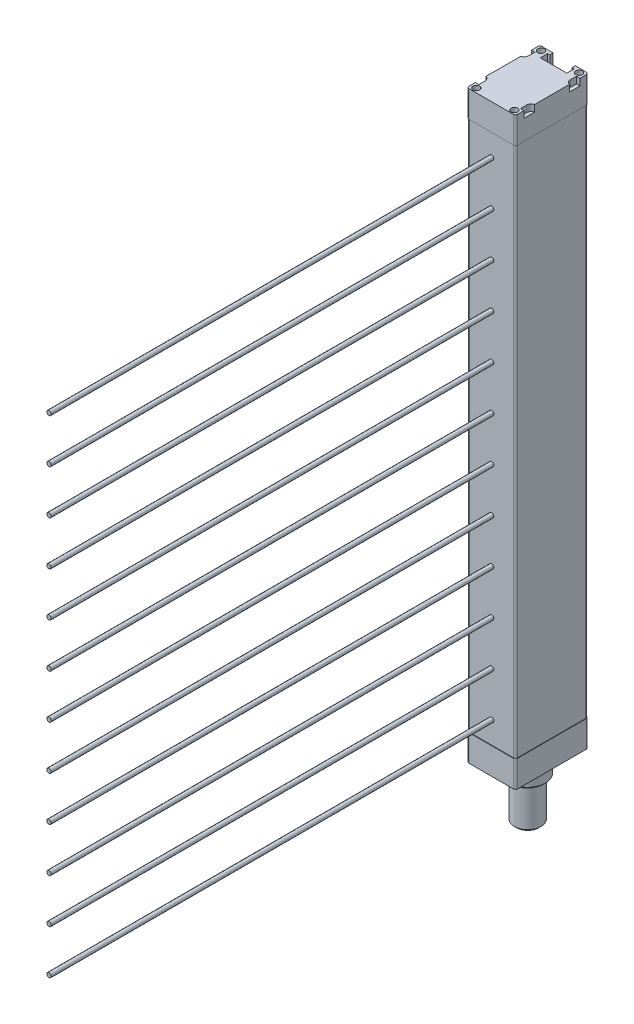
from build123d import *

# Parameters (mm, degrees)
SKETCH_1_R             = 1.5
EXTRUDE_1_DEPTH        = 12
CUT_EXTRUDE_2_DEPTH    = 3
EXTRUDE_3_DEPTH        = 240
SKETCH_5_R             = 1
EXTRUDE_4_DEPTH        = 200
PATTERN_LINEAR_1_COUNT = 12
PATTERN_LINEAR_1_PITCH = 20


with BuildPart() as part:
    # 草圖1 → 伸長1 (new body)
    with BuildSketch(Plane(origin=(0, 0, 0), x_dir=(1, 0, 0), z_dir=(0, 1, 0))):
        with BuildLine():
            Line((-10, 16.5), (-5, 16.5))
            Line((-5, 16.5), (-5, 15))
            Line((-5, 15), (-6, 15))
            Line((-6, 15), (-6, 11.7))
            Line((-6, 11.7), (6, 11.7))
            Line((6, 11.7), (6, 15))
            Line((6, 15), (5, 15))
            Line((5, 15), (5, 16.5))
            Line((5, 16.5), (10, 16.5))
            ThreePointArc((10, 16.5), (10.707106781, 16.207106781), (11, 15.5))
            Line((11, 15.5), (11, -15.5))
            ThreePointArc((11, -15.5), (10.707106781, -16.207106781), (10, -16.5))
            Line((10, -16.5), (-10, -16.5))
            ThreePointArc((-10, -16.5), (-10.707106781, -16.207106781), (-11, -15.5))
            Line((-11, -15.5), (-11, 15.5))
            ThreePointArc((-11, 15.5), (-10.707106781, 16.207106781), (-10, 16.5))
        make_face()
        with Locations(Location((-8.6, 14.6, 0), (0, 0, 270))):
            Circle(SKETCH_1_R, mode=Mode.SUBTRACT)
        with Locations(Location((8.6, 14.6, 0), (0, 0, 90))):
            Circle(SKETCH_1_R, mode=Mode.SUBTRACT)
        with Locations(Location((8.6, -14.6, 0), (0, 0, 270))):
            Circle(SKETCH_1_R, mode=Mode.SUBTRACT)
        with Locations(Location((-8.6, -14.6, 0), (0, 0, 90))):
            Circle(SKETCH_1_R, mode=Mode.SUBTRACT)
    extrude_1 = extrude(amount=EXTRUDE_1_DEPTH)

    # 草圖2 → 伸長2 (cut)
    with BuildSketch(Plane(origin=(0, 12, 0), x_dir=(1, 0, 0), z_dir=(0, 1, 0))):
        with BuildLine():
            Line((-14.2, 12.65), (-9.4, 12.65))
            Line((-9.4, 12.65), (-9.4, 9.85))
            ThreePointArc((-9.4, 9.85), (-9.985786438, 8.435786438), (-11.4, 7.85))
            Line((-11.4, 7.85), (-14.2, 7.85))
            Line((-14.2, 7.85), (-14.2, 12.65))
        make_face()
        with BuildLine():
            Line((9.4, 12.65), (9.4, 9.85))
            ThreePointArc((9.4, 9.85), (9.985786438, 8.435786438), (11.4, 7.85))
            Line((11.4, 7.85), (14.2, 7.85))
            Line((14.2, 7.85), (14.2, 12.65))
            Line((14.2, 12.65), (9.4, 12.65))
        make_face()
        with BuildLine():
            Line((14.2, -12.65), (9.4, -12.65))
            Line((9.4, -12.65), (9.4, -9.85))
            ThreePointArc((9.4, -9.85), (9.985786438, -8.435786438), (11.4, -7.85))
            Line((11.4, -7.85), (14.2, -7.85))
            Line((14.2, -7.85), (14.2, -12.65))
        make_face()
        with BuildLine():
            Line((-9.4, -12.65), (-9.4, -9.85))
            ThreePointArc((-9.4, -9.85), (-9.985786438, -8.435786438), (-11.4, -7.85))
            Line((-11.4, -7.85), (-14.2, -7.85))
            Line((-14.2, -7.85), (-14.2, -12.65))
            Line((-14.2, -12.65), (-9.4, -12.65))
        make_face()
    extrude(amount=-CUT_EXTRUDE_2_DEPTH, mode=Mode.SUBTRACT)

    # 草圖3 → 伸長3 (add)
    with BuildSketch(Plane.XZ):
        with BuildLine():
            Line((-5.2, -16.3), (-5.2, -15.2))
            Line((-5.2, -15.2), (-6.2, -15.2))
            Line((-6.2, -15.2), (-6.2, -11.5))
            Line((-6.2, -11.5), (6.2, -11.5))
            Line((6.2, -11.5), (6.2, -15.2))
            Line((6.2, -15.2), (5.2, -15.2))
            Line((5.2, -15.2), (5.2, -16.3))
            Line((5.2, -16.3), (10, -16.3))
            ThreePointArc((10, -16.3), (10.565685425, -16.065685425), (10.8, -15.5))
            Line((10.8, -15.5), (10.8, 15.5))
            ThreePointArc((10.8, 15.5), (10.565685425, 16.065685425), (10, 16.3))
            Line((10, 16.3), (-10, 16.3))
            ThreePointArc((-10, 16.3), (-10.565685425, 16.065685425), (-10.8, 15.5))
            Line((-10.8, 15.5), (-10.8, -15.5))
            ThreePointArc((-10.8, -15.5), (-10.565685425, -16.065685425), (-10, -16.3))
            Line((-10, -16.3), (-5.2, -16.3))
        make_face()
    extrude(amount=EXTRUDE_3_DEPTH)

    # 鏡射1: 伸長1 across plane
    add(extrude_1.mirror(Plane.ZX.offset(-120)))

    # 草圖4 → 旋轉1 (revolve)
    with BuildSketch(Plane(origin=(0, 0, 0), x_dir=(0, 0, -1), z_dir=(1, 0, 0))):
        Polygon((8, -252), (8, -259), (7, -259), (7, -260), (6, -260), (6, -277), (5, -278), (0, -278), (0, -252), align=None)
    revolve(axis=Axis((0, -252, 0), (0, 1, 0)))

    # 草圖5 → 伸長4 (add)
    with BuildSketch(Plane.XY.offset(16.3)):
        with Locations(Location((0, -10, 0), (0, 0, 180))):
            Circle(SKETCH_5_R)
    extrude_4 = extrude(amount=EXTRUDE_4_DEPTH)

    # 阵列(线性)1: 伸長4 ×12
    with Locations(*[(0, -i * PATTERN_LINEAR_1_PITCH, 0) for i in range(1, PATTERN_LINEAR_1_COUNT)]):
        add(extrude_4)


solid = part.part
